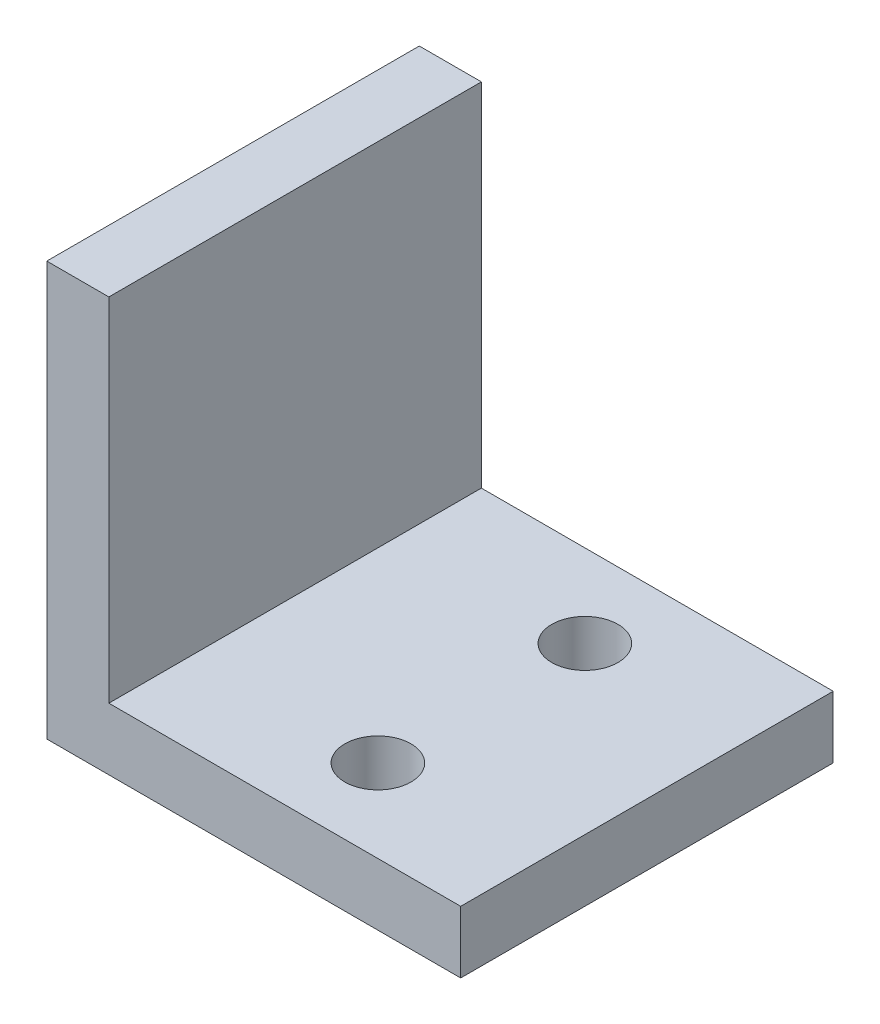
SolidWorks part; units mm, degrees
material "AISI 1015 钢，冷拔 (SS)"
ref_plane "Front Plane" through (0, 0, 0) normal (0, 0, 1) x (1, 0, 0)
ref_plane "Top Plane" through (0, 0, 0) normal (0, 1, 0) x (1, 0, 0)
ref_plane "Right Plane" through (0, 0, 0) normal (1, 0, 0) x (0, 0, -1)
other "Configuration Table"
sketch "Sketch1" plane through (0, 0, 0) normal (0, 0, 1) x (1, 0, 0)
  line L0 (0, 0) -> (0, 100)
  line L1 (0, 100) -> (15, 100)
  line L2 (15, 100) -> (15, 15)
  line L3 (15, 15) -> (100, 15)
  line L4 (100, 15) -> (100, 0)
  line L5 (100, 0) -> (0, 0)
  dimension "D1" = 100
  dimension "D2" = 100
  dimension "D3" = 15
  dimension "D4" = 15
extrude "Boss-Extrude1" add sketch "Sketch1" along normal blind 90
sketch "Sketch2" plane through (0, 15, 0) normal (0, 1, 0) x (1, 0, 0)
  line L0 (100, -90) -> (100, 0) construction
  line L1 (100, 0) -> (15, 0) construction
  circle A0 centre (60, -20) radius 8
  circle A1 centre (60, -70) radius 8
  dimension "D1" = 16
  dimension "D2" = 16
  dimension "D3" = 40
  dimension "D4" = 50
  dimension "D5" = 20
extrude "Cut-Extrude1" cut sketch "Sketch2" against normal blind 90
